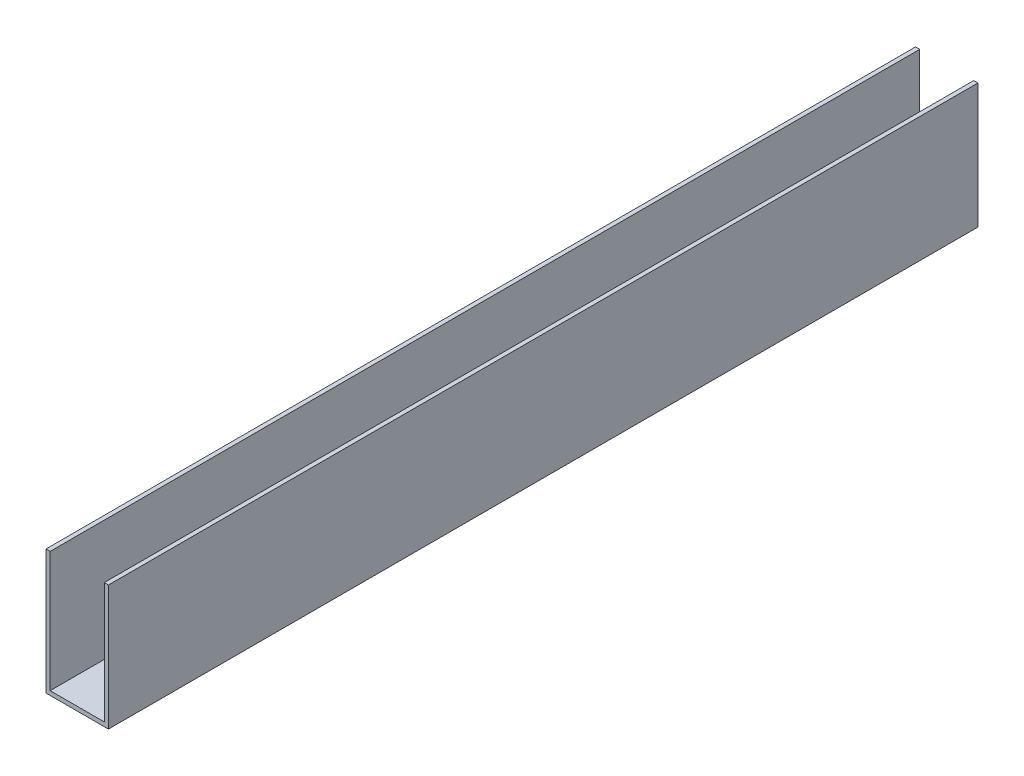
SolidWorks part; units mm, degrees
material "标准件"
ref_plane "前视基准面" through (0, 0, 0) normal (0, 0, 1) x (1, 0, 0)
ref_plane "上视基准面" through (0, 0, 0) normal (0, 1, 0) x (1, 0, 0)
ref_plane "右视基准面" through (0, 0, 0) normal (1, 0, 0) x (0, 0, -1)
sketch "草图1" plane through (0, 0, 0) normal (0, 0, 1) x (1, 0, 0)
  line L0 (0, 0) -> (0, 33.955) construction
  line L2 (-15, -30) -> (15, -30)
  line L3 (-15, -30) -> (-15, 30)
  line L4 (-15, 30) -> (15, 30)
  line L5 (15, -30) -> (15, 30)
  line L6 (-15, -30) -> (15, 30) construction
  line L7 (-15, 30) -> (15, -30) construction
  dimension "D1" = 30
  dimension "D2" = 60
extrude "凸台-拉伸1" add sketch "草图1" along normal mid plane 418
shell "抽壳1" thickness 2
